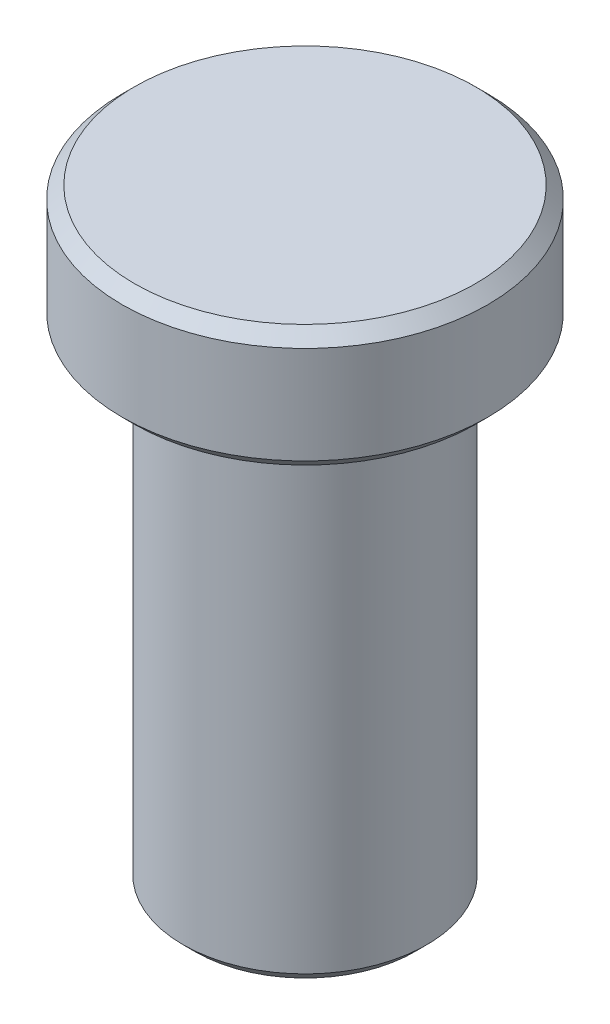
from build123d import *

# Parameters (mm, degrees)
SKETCH2_R           = 5
BOSS_EXTRUDE1_DEPTH = 20
SKETCH3_R           = 7.5
BOSS_EXTRUDE2_DEPTH = 5
CHAMFER2_SIZE       = 0.5


with BuildPart() as part:
    # Sketch2 → Boss-Extrude1 (new body)
    with BuildSketch(Plane(origin=(0, 0, 0), x_dir=(1, 0, 0), z_dir=(0, 1, 0))):
        with Locations(Location((0, 0, 0), (0, 0, 270))):
            Circle(SKETCH2_R)
    extrude(amount=BOSS_EXTRUDE1_DEPTH)

    # Sketch3 → Boss-Extrude2 (add)
    with BuildSketch(Plane(origin=(0, 20, 0), x_dir=(1, 0, 0), z_dir=(0, 1, 0))):
        with Locations(Location((0, 0, 0), (0, 0, 270))):
            Circle(SKETCH3_R)
    extrude(amount=BOSS_EXTRUDE2_DEPTH)

    # Chamfer2
    chamfer2_edges = [part.edges().sort_by_distance(p)[0] for p in [
        (0, 0, -5),
        (0, 20, -7.5),
        (0, 25, -7.5),
    ]]
    chamfer(chamfer2_edges, length=CHAMFER2_SIZE)


solid = part.part
